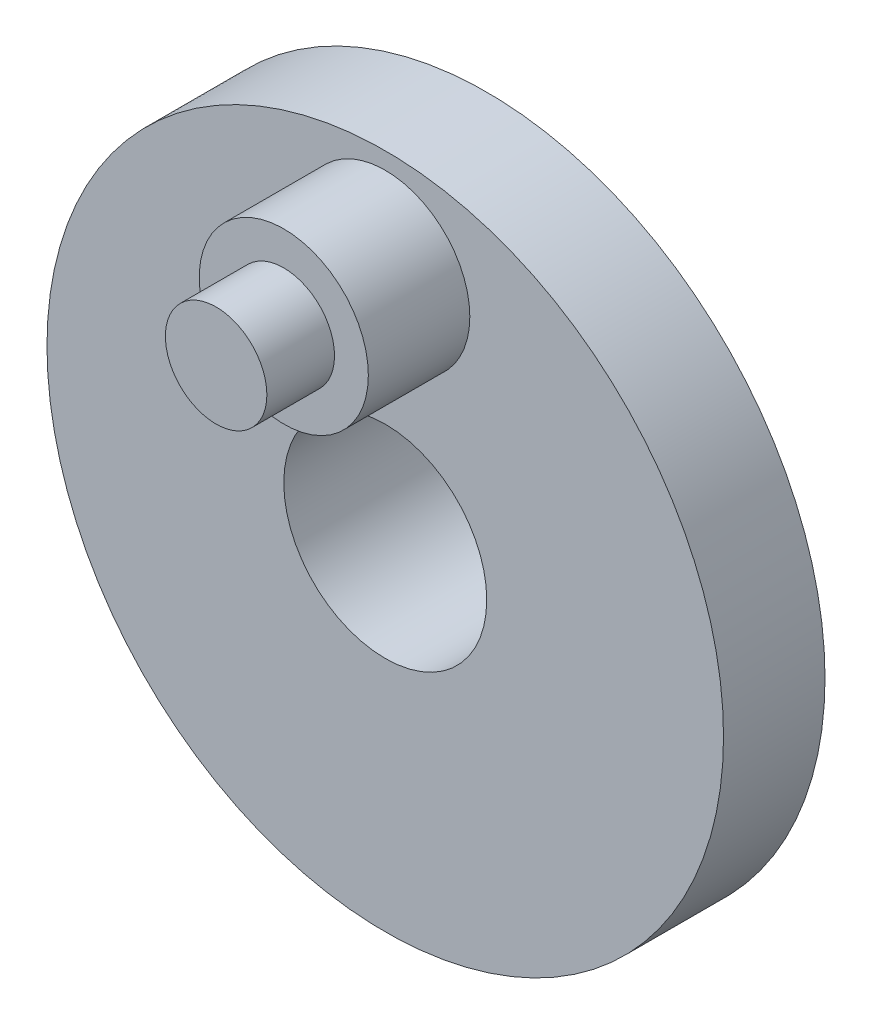
SolidWorks part; units mm, degrees
ref_plane "Front Plane" through (0, 0, 0) normal (0, 0, 1) x (1, 0, 0)
ref_plane "Top Plane" through (0, 0, 0) normal (0, 1, 0) x (1, 0, 0)
ref_plane "Right Plane" through (0, 0, 0) normal (1, 0, 0) x (0, 0, -1)
sketch "Sketch1" plane through (0, 0, 0) normal (0, 0, 1) x (1, 0, 0)
  circle A0 centre (0, 0) radius 10
  dimension "D1" = 20
extrude "Boss-Extrude1" add sketch "Sketch1" along normal blind 3
sketch "Sketch2" plane through (0, 0, 3) normal (0, 0, 1) x (1, 0, 0)
  circle A0 centre (0, 7) radius 2.5
  dimension "D2" = 5
  dimension "D1" = 7
extrude "Boss-Extrude2" add sketch "Sketch2" along normal blind 3
sketch "Sketch3" plane through (0, 0, 6) normal (0, 0, 1) x (1, 0, 0)
  circle A0 centre (0, 7) radius 1.5
  dimension "D1" = 3
extrude "Boss-Extrude3" add sketch "Sketch3" along normal blind 2
sketch "Sketch4" plane through (0, 0, 0) normal (0, 0, -1) x (-1, 0, 0)
  circle A0 centre (0, 0) radius 3
  dimension "D1" = 6
extrude "Cut-Extrude1" cut sketch "Sketch4" against normal blind 24
sketch "Sketch5" plane through (0, 0, 0) normal (0, 0, -1) x (-1, 0, 0)
  circle A0 centre (0, 0) radius 3
  circle A1 centre (0, 0) radius 4
  dimension "D1" = 8
  dimension "D2" = 6
extrude "Boss-Extrude4" add sketch "Sketch5" along normal blind 4
sketch "Sketch6" plane through (0, 0, 0) normal (1, 0, 0) x (0, 0, -1)
  circle A0 centre (2, 0) radius 1
  dimension "D1" = 2
extrude "Cut-Extrude2" cut sketch "Sketch6" against normal mid plane 10
